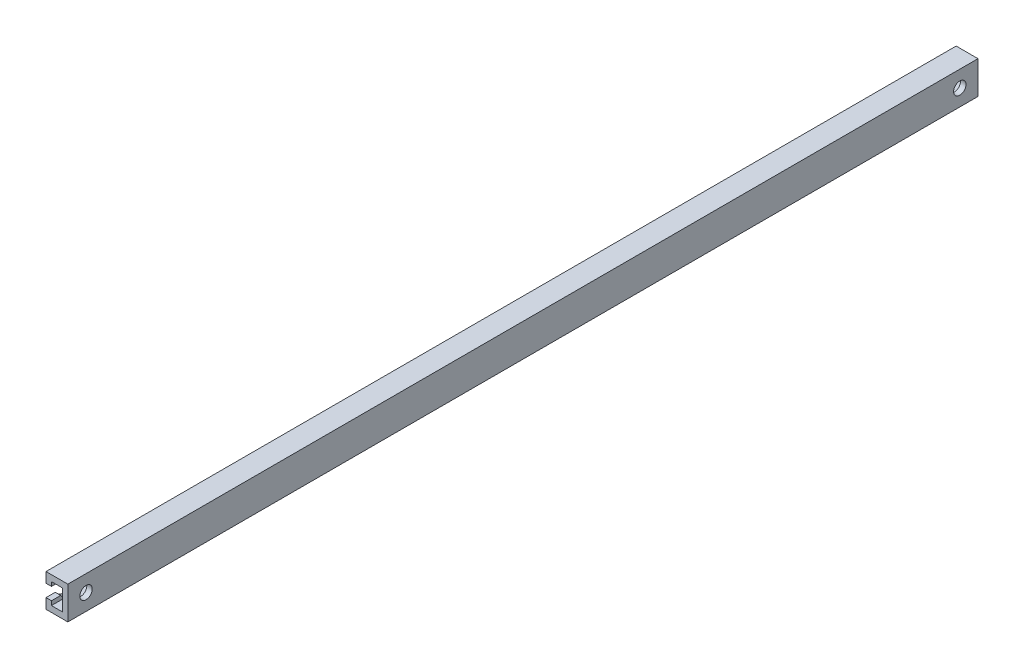
SolidWorks part; units mm, degrees
ref_plane "前基準面" through (0, 0, 0) normal (0, 0, 1) x (1, 0, 0)
ref_plane "上基準面" through (0, 0, 0) normal (0, 1, 0) x (1, 0, 0)
ref_plane "右基準面" through (0, 0, 0) normal (1, 0, 0) x (0, 0, -1)
sketch "草圖1" plane through (0, 0, 0) normal (0, 0, 1) x (1, 0, 0)
  line L0 (3, 4.5) -> (-3, -4.5) construction
  line L1 (-3, 4.5) -> (3, 4.5)
  line L2 (-3, 4.5) -> (-3, 1.7)
  line L3 (-3, -4.5) -> (3, -4.5)
  line L4 (3, 4.5) -> (3, -4.5)
  line L5 (-3.5323, 0) -> (3.7285, 0) construction
  line L6 (-3, 1.7) -> (-1.5, 1.7)
  line L7 (-3, -1.7) -> (-1.5, -1.7)
  line L8 (-1.5, 1.7) -> (-1.5, 2.85)
  line L9 (-1.5, 2.85) -> (1.5, 2.85)
  line L10 (-1.5, -2.85) -> (1.5, -2.85)
  line L11 (-1.5, -1.7) -> (-1.5, -2.85)
  line L12 (-3, -1.7) -> (-3, -4.5)
  line L13 (1.5, 2.85) -> (1.5, -2.85)
  dimension "D1" = 6
  dimension "D2" = 9
  dimension "D3" = 3.4
  dimension "D4" = 1.5
  dimension "D5" = 3
  dimension "D6" = 5.7
extrude "伸長1" add sketch "草圖1" along normal blind 250
hole_wizard "打孔尺寸(%根据)内六角圆柱头螺钉的类型1" positions "草圖3" profile "草圖2" counterbore size "M3" standard "GB" end condition through all
sketch "草圖3" plane through (-3, 0, 0) normal (-1, 0, 0) x (0, 0, 1)
  line L0 (250, 4.5) -> (0, 4.5) construction
  line L1 (250, 2.85) -> (250, -2.85) construction
  line L2 (0, -1.7) -> (0, -4.5) construction
  point P0 (245, 0)
  point P5 (5, 0)
  dimension "D1" = 4.5
  dimension "D2" = 5
  dimension "D3" = 5
sketch "草圖2" plane through (-3, 0, 245) normal (0, 1, 0) x (0, 0, 1)
  line L0 (0, 0) -> (0, 6)
  line L1 (0, 6) -> (1.7, 6)
  line L3 (1.7, 6) -> (1.7, 3.4)
  line L4 (1.7, 3.4) -> (3, 3.4)
  line L5 (3, 3.4) -> (3, 0)
  line L7 (3, 0) -> (0, 0)
  line L11 (0, -6.35) -> (0, 107.95) construction
  dimension "通孔孔直径" = 3.4
  dimension "通孔孔深度" = 6
  dimension "柱形沉头孔直径" = 6
  dimension "柱形沉头孔深度" = 3.4
